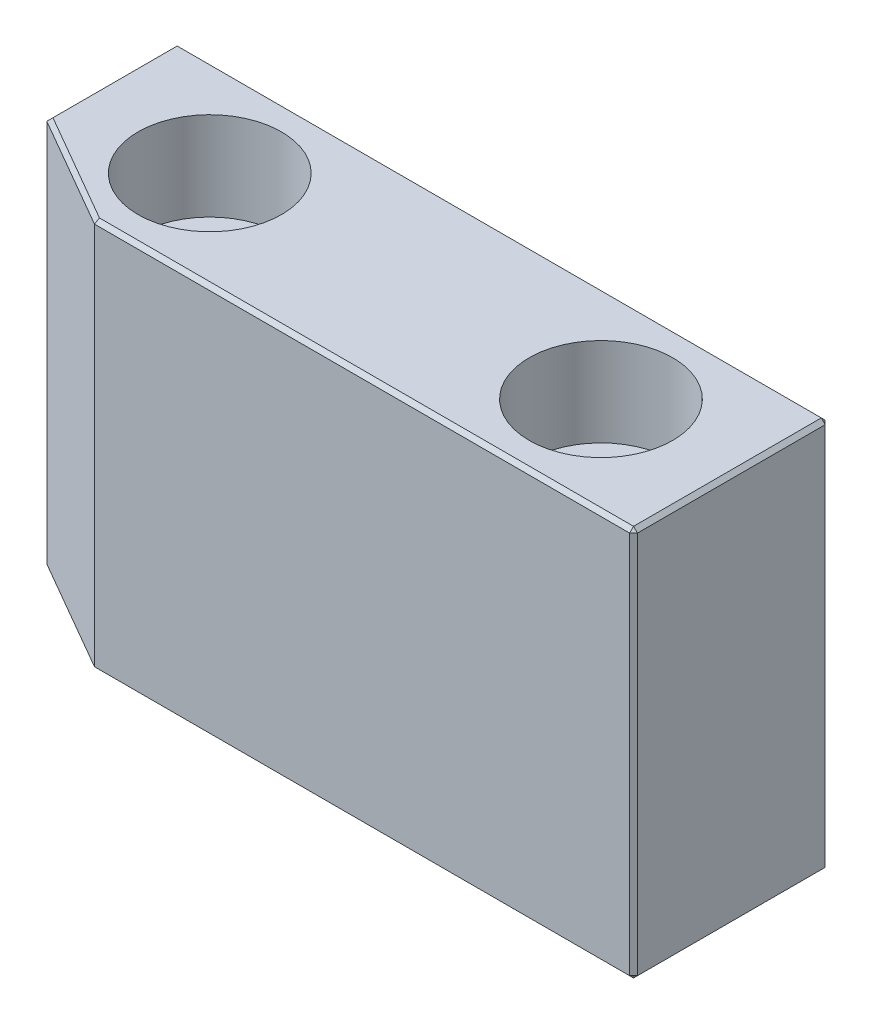
from build123d import *

# Parameters (mm, degrees)
SKETCH_1_W                = 50
SKETCH_1_H                = 30
EXTRUDE_1_DEPTH           = 15
HOLE_WIZARD_1_D           = 6.6
HOLE_WIZARD_1_CBORE_D     = 11
HOLE_WIZARD_1_CBORE_DEPTH = 6.8
CHAMFER_1_SIZE            = 5
CHAMFER_1_SIZE2           = 8.660254038
CHAMFER_2_SIZE            = 0.3


with BuildPart() as part:
    # 草图1 → 凸台-拉伸1 (new body)
    with BuildSketch(Plane.XY):
        Rectangle(SKETCH_1_W, SKETCH_1_H)
    extrude(amount=EXTRUDE_1_DEPTH)

    # 打孔尺寸根据内六角圆柱头螺钉的类型1 (through all)
    with Locations(Plane(origin=(0, 15, 0), x_dir=(1, 0, 0), z_dir=(0, 1, 0))):
        with Locations((-15, -7.5), (15, -7.5)):
            CounterBoreHole(HOLE_WIZARD_1_D / 2, HOLE_WIZARD_1_CBORE_D / 2, HOLE_WIZARD_1_CBORE_DEPTH)

    # 倒角1
    chamfer_1_edges = [part.edges().sort_by_distance(p)[0] for p in [
        (-25, 0, 15),
    ]]
    chamfer_1_side = [part.faces().sort_by_distance(p)[0] for p in [
        (-25, 0, 7.5),
    ]]
    chamfer(chamfer_1_edges, length=CHAMFER_1_SIZE, length2=CHAMFER_1_SIZE2, reference=chamfer_1_side[0])

    # 倒角2
    chamfer_2_edges = [part.edges().sort_by_distance(p)[0] for p in [
        (4.330127019, -15, 15),
        (-25, -15, 5),
        (-20.669872981, -15, 12.5),
        (-25, 15, 5),
        (-20.669872981, 15, 12.5),
        (25, 0, 15),
        (0, -15, 0),
        (-25, 0, 0),
        (0, 15, 0),
        (25, 0, 0),
        (4.330127019, 15, 15),
        (25, -15, 7.5),
        (25, 15, 7.5),
    ]]
    chamfer(chamfer_2_edges, length=CHAMFER_2_SIZE)


solid = part.part
